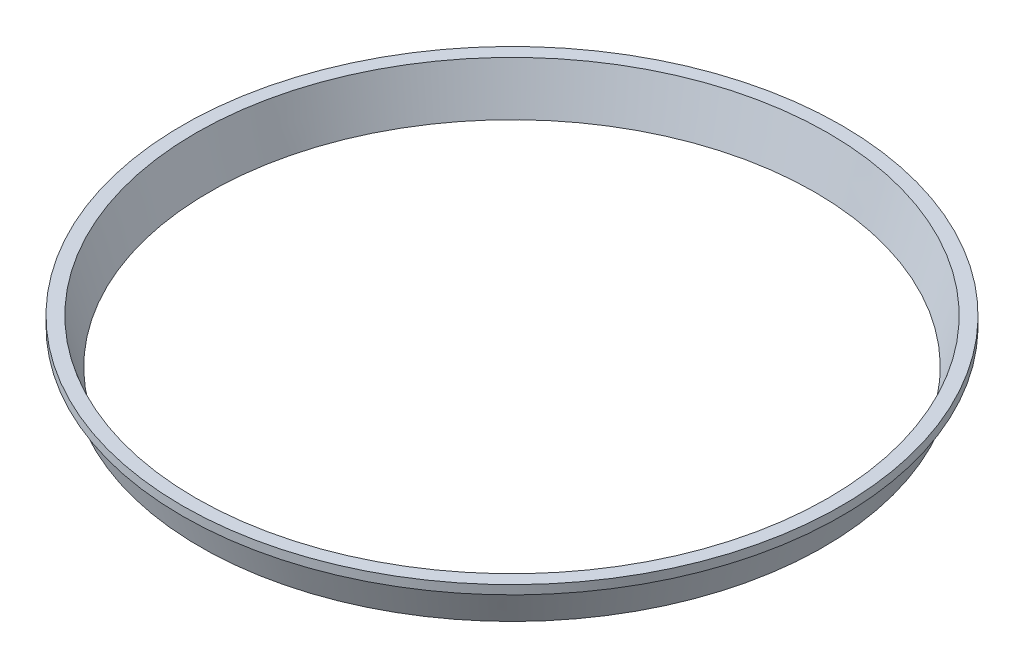
from build123d import *


with BuildPart() as part:
    # Sketch 5 → Revolve 1 (revolve)
    with BuildSketch(Plane.XY, mode=Mode.PRIVATE) as revolve_1_sk:
        Polygon((-68, 0), (-71, 10), (-74, 10), (-74, 8), (-72.4, 8), (-70, 0), align=None)
    revolve(revolve_1_sk.sketch.rotate(Axis((0, 0, 0), (0, 1, 0)), 270), axis=Axis((0, 0, 0), (0, 1, 0)))


solid = part.part
